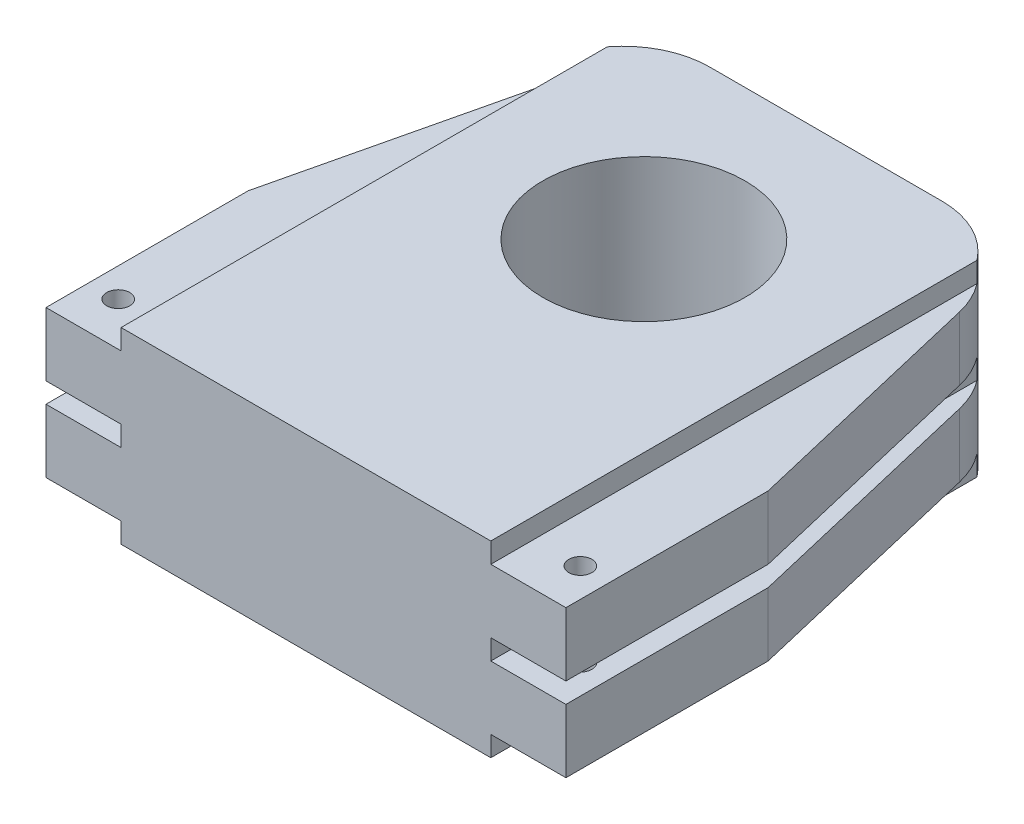
SolidWorks part; units mm, degrees
material "普通碳钢"
ref_plane "Front Plane" through (0, 0, 0) normal (0, 0, 1) x (1, 0, 0)
ref_plane "Top Plane" through (0, 0, 0) normal (0, 1, 0) x (1, 0, 0)
ref_plane "Right Plane" through (0, 0, 0) normal (1, 0, 0) x (0, 0, -1)
other "Configuration Table"
sketch "Sketch1" plane through (0, 0, 0) normal (0, 1, 0) x (1, 0, 0)
  line L0 (-90, 0) -> (90, 0)
  line L1 (-40.25, 180) -> (40.25, 180)
  line L2 (-90, 0) -> (-90, 70)
  line L3 (90, 0) -> (90, 70)
  line L4 (-40.25, 180) -> (-40.25, 150) construction
  line L5 (-40.25, 150) -> (-70.25, 150) construction
  line L6 (-90, 70) -> (-69.4445, 156.9053)
  line L7 (0, 0) -> (0, 88.5903) construction
  line L8 (90, 70) -> (69.4445, 156.9053)
  arc A0 (-40.25, 180) -> (-69.4445, 156.9053) centre (-40.25, 150) ccw
  arc A1 (40.25, 180) -> (69.4445, 156.9053) centre (40.25, 150) cw
  point P4 (0, 0)
  point P7 (0, 180)
  dimension "D1" = 180
  dimension "D2" = 80.5
  dimension "D3" = 180
  dimension "D4" = 70
  dimension "D5" = 30
extrude "Boss-Extrude1" add sketch "Sketch1" along normal blind 65
sketch "Sketch2" plane through (0, 65, 0) normal (0, 1, 0) x (1, 0, 0)
  line L0 (40.25, 180) -> (-40.25, 180) construction
  circle A0 centre (0, 117) radius 35
  dimension "D1" = 70
  dimension "D2" = 63
extrude "Cut-Extrude1" cut sketch "Sketch2" against normal blind 65
sketch "Sketch3" plane through (0, 0, 0) normal (0, 0, 1) x (1, 0, 0)
  line L1 (90, 0) -> (64, 0)
  line L2 (90, 0) -> (90, 7)
  line L3 (90, 7) -> (64, 7)
  line L4 (64, 0) -> (64, 7)
  line L5 (90, 65) -> (64, 65)
  line L6 (90, 65) -> (90, 58)
  line L7 (90, 58) -> (64, 58)
  line L8 (64, 65) -> (64, 58)
  line L9 (-90, 65) -> (-64, 65)
  line L10 (-90, 65) -> (-90, 58)
  line L11 (-90, 58) -> (-64, 58)
  line L12 (-64, 65) -> (-64, 58)
  line L13 (-90, 0) -> (-64, 0)
  line L14 (-90, 0) -> (-90, 7)
  line L15 (-90, 7) -> (-64, 7)
  line L16 (-64, 0) -> (-64, 7)
  dimension "D1" = 26
  dimension "D2" = 7
  dimension "D3" = 26
  dimension "D4" = 7
  dimension "D5" = 26
  dimension "D6" = 7
  dimension "D7" = 7
  dimension "D8" = 26
extrude "Cut-Extrude2" cut sketch "Sketch3" against normal through all
sketch "Sketch4" plane through (0, 7, 0) normal (0, -1, 0) x (1, 0, 0)
  line L0 (90, -70) -> (90, 0) construction
  line L1 (90, 0) -> (64, 0) construction
  line L2 (-90, -70) -> (-90, 0) construction
  circle A0 centre (80, -15) radius 4
  circle A1 centre (-80, -15) radius 4
  dimension "D1" = 8
  dimension "D2" = 8
  dimension "D3" = 10
  dimension "D4" = 15
  dimension "D5" = 10
extrude "Cut-Extrude3" cut sketch "Sketch4" against normal through all
sketch "Sketch5" plane through (0, 0, 0) normal (0, 0, 1) x (1, 0, 0)
  line L0 (-90, 58) -> (-90, 7) construction
  line L1 (-90, 36) -> (-64, 36)
  line L2 (-90, 36) -> (-90, 29)
  line L3 (-90, 29) -> (-64, 29)
  line L4 (-64, 36) -> (-64, 29)
  line L5 (90, 58) -> (90, 7) construction
  line L6 (90, 36) -> (64, 36)
  line L7 (90, 36) -> (90, 29)
  line L8 (90, 29) -> (64, 29)
  line L9 (64, 36) -> (64, 29)
  line L10 (-90, 58) -> (-64, 58) construction
  line L11 (64, 58) -> (90, 58) construction
  dimension "D1" = 7
  dimension "D2" = 26
  dimension "D3" = 26
  dimension "D4" = 7
  dimension "D5" = 22
  dimension "D6" = 22
extrude "Cut-Extrude4" cut sketch "Sketch5" against normal through all
